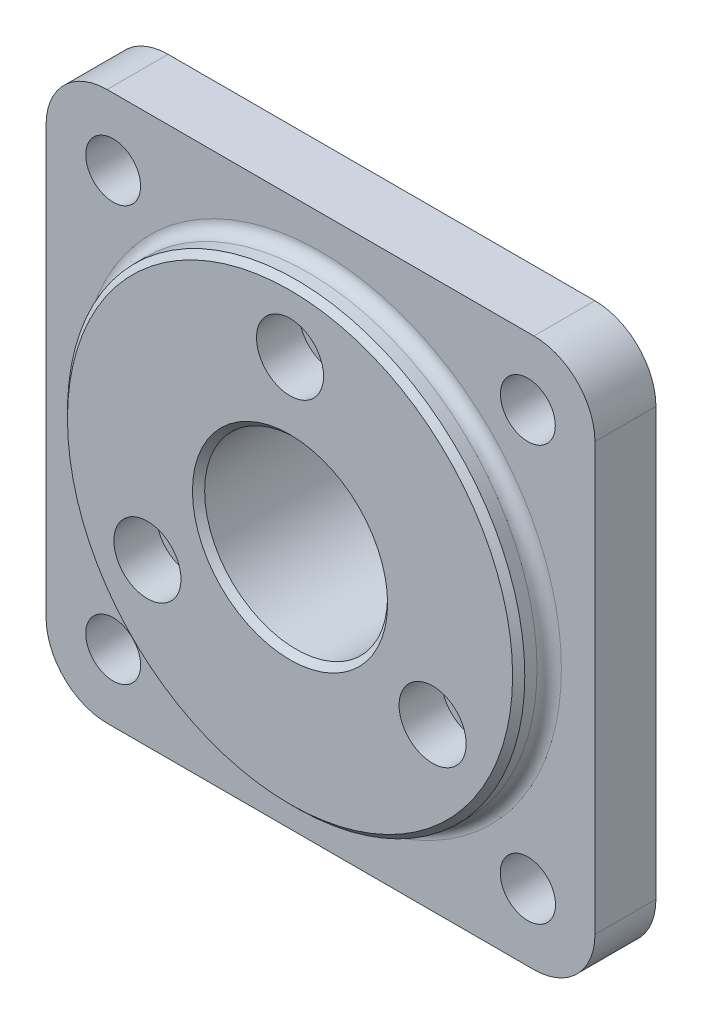
SolidWorks part; units mm, degrees
ref_plane "前视基准面" through (0, 0, 0) normal (0, 0, 1) x (1, 0, 0)
ref_plane "上视基准面" through (0, 0, 0) normal (0, 1, 0) x (1, 0, 0)
ref_plane "右视基准面" through (0, 0, 0) normal (1, 0, 0) x (0, 0, -1)
sketch "草图1" plane through (0, 0, 0) normal (0, 0, 1) x (1, 0, 0)
  line L1 (-45, 45) -> (45, 45)
  line L2 (-45, 45) -> (-45, -45)
  line L3 (-45, -45) -> (45, -45)
  line L4 (45, 45) -> (45, -45)
  line L5 (-45, 45) -> (45, -45) construction
  line L6 (-45, -45) -> (45, 45) construction
  point P0 (0, 0)
  dimension "D1" = 90
  dimension "D2" = 90
extrude "凸台-拉伸1" add sketch "草图1" along normal blind 10
fillet "圆角1" radius 10 4 edges at (-45, -45, 5) (45, -45, 5) (45, 45, 5) (-45, 45, 5)
sketch "草图2" plane through (0, 0, 10) normal (0, 0, 1) x (1, 0, 0)
  line L1 (-34, 34) -> (34, 34) construction
  line L2 (-34, 34) -> (-34, -34) construction
  line L3 (-34, -34) -> (34, -34) construction
  line L4 (34, 34) -> (34, -34) construction
  line L5 (-34, 34) -> (34, -34) construction
  line L6 (-34, -34) -> (34, 34) construction
  circle A0 centre (-34, 34) radius 4.5
  circle A1 centre (34, 34) radius 4.5
  circle A2 centre (-34, -34) radius 4.5
  circle A3 centre (34, -34) radius 4.53
  point P0 (0, 0)
  dimension "D1" = 68
  dimension "D2" = 68
extrude "切除-拉伸1" cut sketch "草图2" against normal through all
sketch "草图3" plane through (0, 0, 10) normal (0, 0, 1) x (1, 0, 0)
  circle A0 centre (0, 0) radius 37.5
extrude "凸台-拉伸2" add sketch "草图3" along normal blind 5
sketch "草图4" plane through (0, 0, 0) normal (0, 0, -1) x (-1, 0, 0)
  circle A0 centre (0, 0) radius 17.5
extrude "凸台-拉伸3" add sketch "草图4" along normal blind 7
sketch "草图5" plane through (0, 0, 15) normal (0, 0, 1) x (1, 0, 0)
  circle A0 centre (0, 0) radius 15
extrude "切除-拉伸2" cut sketch "草图5" against normal through all
sketch "草图6" plane through (0, 0, 15) normal (0, 0, 1) x (1, 0, 0)
  line L0 (0, 42.6092) -> (0, 0) construction
  circle A0 centre (0, 27) radius 5.5
  dimension "D2" = 11
  dimension "D1" = 27
extrude "切除-拉伸3" cut sketch "草图6" against normal blind 7
sketch "草图7" plane through (0, 0, 8) normal (0, 0, 1) x (1, 0, 0)
  circle A0 centre (0, 27) radius 3.5
extrude "切除-拉伸4" cut sketch "草图7" against normal through all
pattern_circular "阵列(圆周)1" count 3 over 360 about axis through (0, 0, 0) along (0, 0, 1) of "切除-拉伸4", "切除-拉伸3"
fillet "圆角2" radius 2 1 edges at (37.5, 0, 10)
chamfer "倒角1" distance 1 angle 45 3 edges at (-17.5, 0, -7) (15, 0, 15) (37.5, 0, 15)
